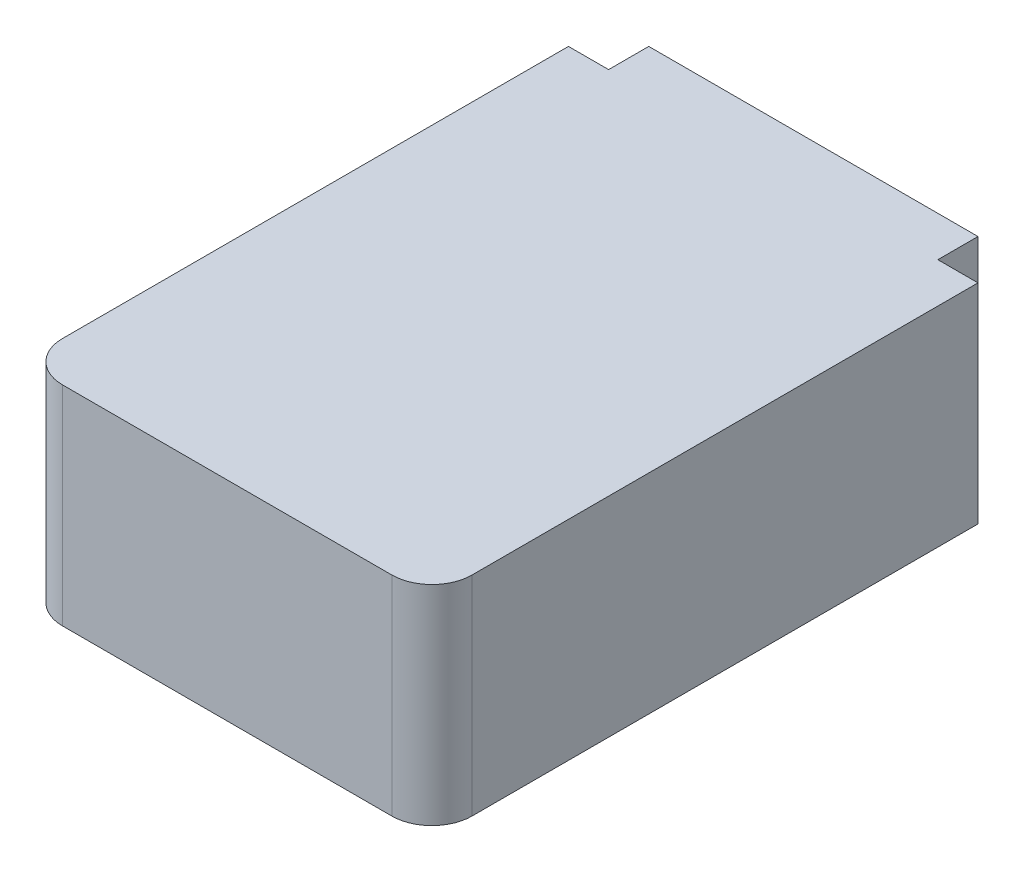
SolidWorks part; units mm, degrees
ref_plane "前视基准面" through (0, 0, 0) normal (0, 0, 1) x (1, 0, 0)
ref_plane "上视基准面" through (0, 0, 0) normal (0, 1, 0) x (1, 0, 0)
ref_plane "右视基准面" through (0, 0, 0) normal (1, 0, 0) x (0, 0, -1)
sketch "草图1" plane through (0, 0, 0) normal (0, 1, 0) x (1, 0, 0)
  line L1 (-25.5, 36.5) -> (25.5, 36.5)
  line L2 (-25.5, 36.5) -> (-25.5, -36.5)
  line L3 (-25.5, -36.5) -> (25.5, -36.5)
  line L4 (25.5, 36.5) -> (25.5, -36.5)
  line L5 (-25.5, 36.5) -> (25.5, -36.5) construction
  line L6 (-25.5, -36.5) -> (25.5, 36.5) construction
  point P0 (0, 0)
  dimension "D1" = 51
  dimension "D2" = 73
extrude "凸台-拉伸1" add sketch "草图1" along normal blind 26
fillet "圆角1" radius 5 4 edges at (25.5, 13, 36.5) (25.5, 13, -36.5) (-25.5, 13, -36.5) (-25.5, 13, 36.5)
sketch "草图2" plane through (0, 0, 0) normal (0, -1, 0) x (1, 0, 0)
  line L0 (20.5, -36.5) -> (-20.5, -36.5) construction
  line L1 (25.5, -36.5) -> (20.5, -36.5)
  line L2 (25.5, -36.5) -> (25.5, -31.5)
  line L3 (25.5, -31.5) -> (20.5, -31.5)
  line L4 (20.5, -36.5) -> (20.5, -31.5)
  line L5 (25.5, 31.5) -> (25.5, -31.5) construction
  line L6 (-25.5, -36.5) -> (-20.5, -36.5)
  line L7 (-25.5, -36.5) -> (-25.5, -31.5)
  line L8 (-25.5, -31.5) -> (-20.5, -31.5)
  line L9 (-20.5, -36.5) -> (-20.5, -31.5)
  line L10 (-25.5, -31.5) -> (-25.5, 31.5) construction
  dimension "D1" = 5
  dimension "D2" = 5
  dimension "D3" = 0
  dimension "D4" = 5
  dimension "D5" = 5
  dimension "D6" = 0
extrude "切除-拉伸1" cut sketch "草图2" against normal blind 30
hole_wizard "M3 螺纹孔1" positions "草图3" profile "草图4" tap size "M3" standard "GB"
sketch "草图3" plane through (0, 0, 0) normal (0, -1, 0) x (-1, 0, 0)
  line L0 (-20.5, 36.5) -> (20.5, 36.5) construction
  line L3 (-25.5, -31.5) -> (-25.5, 31.5) construction
  point P0 (14.8, -8.3)
  point P2 (-16.2, -8.3)
  point P4 (14.8, 21.7)
  point P6 (-16.2, 21.7)
  dimension "D1" = 30
  dimension "D2" = 31
  dimension "D3" = 14.8
  dimension "D4" = 9.3
cosmetic thread "孔螺蚊线1" parameters "D1"=6, "D2"=3
cosmetic thread "孔螺蚊线2" parameters "D1"=6, "D2"=3
cosmetic thread "孔螺蚊线3" parameters "D1"=6, "D2"=3
cosmetic thread "孔螺蚊线4" parameters "D1"=6, "D2"=3
sketch "草图4" plane through (-14.8, 0, 8.3) normal (1, 0, 0) x (0, 0, -1)
  line L0 (0, 0) -> (0, 8.2511)
  line L1 (0, 8.2511) -> (1.25, 7.5)
  line L2 (1.25, 7.5) -> (1.25, 0)
  line L5 (1.25, 0) -> (0, 0)
  line L10 (0, 8.2511) -> (-1.25, 7.5) construction
  line L11 (0, -6.35) -> (0, 107.95) construction
  dimension "螺纹孔钻头直径" = 2.5
  dimension "螺纹孔钻头深度" = 7.5
  dimension "导头角度" = 118
